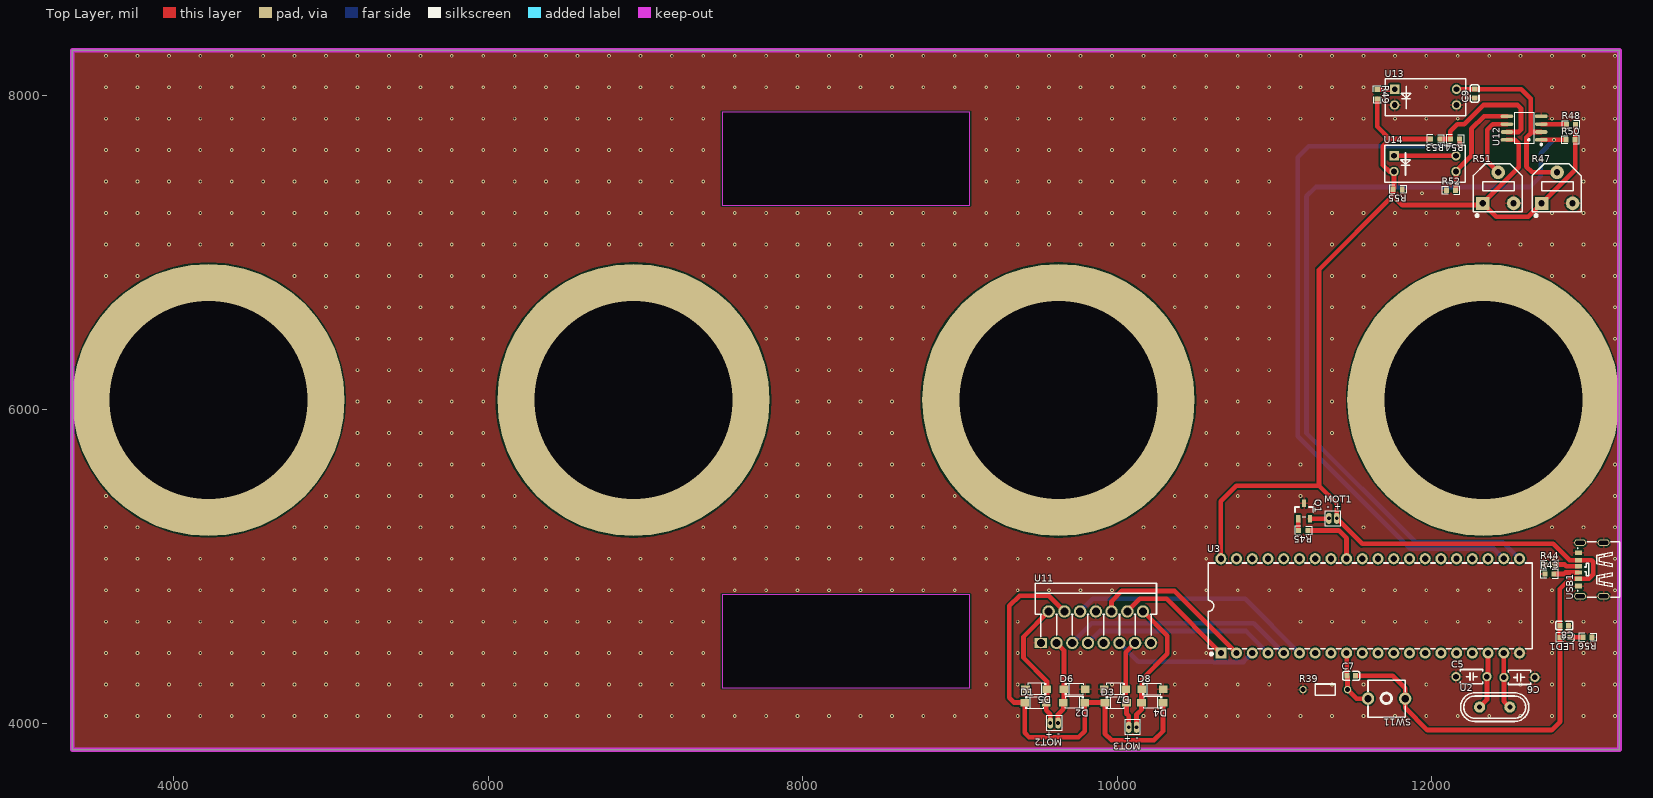
[diagram p0: Top Layer view]
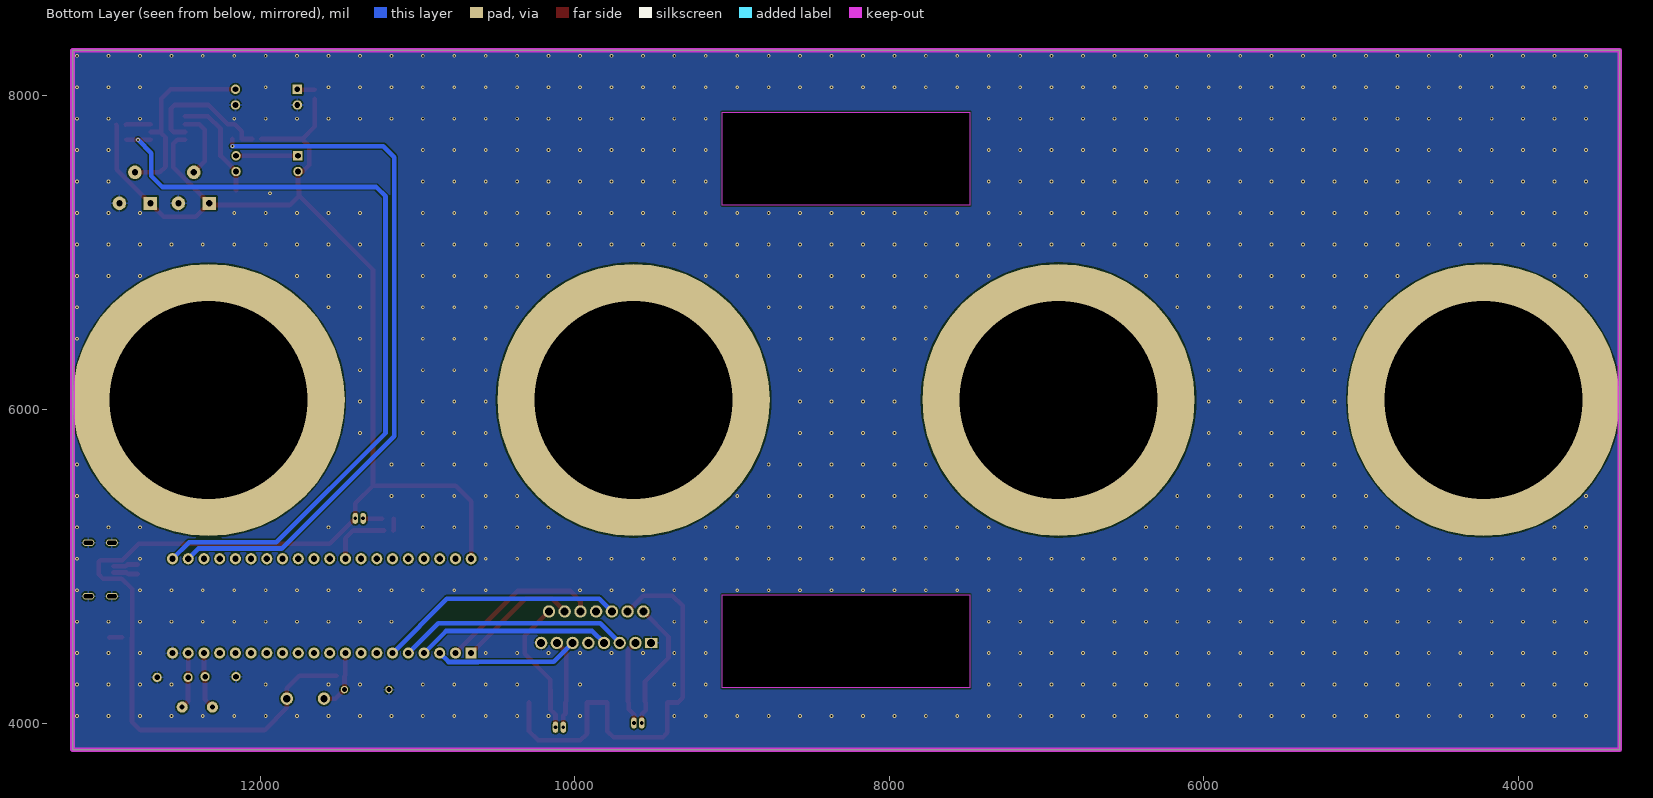
[diagram p1: Bottom Layer view, seen from below]
# Altium PCB MISC61231.pcbdoc
Units mil, origin at the board's own origin, x right, y up, seen from the top; angles counter-clockwise.
Board outline 9842.52 x 4448.82 mil, 2 copper layers (Top Layer, Bottom Layer), stack 62.206 mil thick; 40 components, 32 nets, 156 pads, 697 vias.

## Layer stack, top to bottom
Top Solder Mask Layer: solder mask 0.394, Dk 3.3
Top Layer: signal copper 1.379
SUBSTRATE1: surface 59.449, FR4, Dk 4.5
Bottom Layer: signal copper 1.378
Bottom Solder Mask Layer: solder mask 0.394, Dk 3.3

## Board outline
3353.74,8284.41 3353.74,3835.59 13196.26,3835.59 13196.26,8284.41
cut-out: 7487.6,7890.71 7487.6,7300.16 9062.4,7300.16 9062.4,7890.71
cut-out: 9062.4,4229.29 9062.4,4819.84 7487.6,4819.84 7487.6,4229.29

## Design rules (kind name [scope] priority, off if disabled: settings)
BoardOutlineClearance copperThickness2oz_1 [All] p2 off: genericclearance=7.99 ignorepadtopadclearanceinfootprint=FALSE except(0: Arc-SplitContinuation Track-SplitContinuation SMDPad-SplitContinuation THPad-SplitContinuation Via-SplitContinuation Fill-SplitContinuation Region-SplitContinuation Poly-SplitContinuation Text-SplitContinuation Hole-SplitContinuation; 5.98: Arc-CutoutEdge Track-CutoutEdge SMDPad-CutoutEdge THPad-CutoutEdge Via-CutoutEdge Text-CutoutEdge; 6.9: Hole-OutlineEdge Hole-CutoutEdge; 10: Poly-OutlineEdge Poly-CutoutEdge; 11.81: Arc-OutlineEdge Track-OutlineEdge SMDPad-OutlineEdge THPad-OutlineEdge Via-OutlineEdge Fill-OutlineEdge Region-OutlineEdge Text-OutlineEdge Fill-CutoutEdge Region-CutoutEdge)
BoardOutlineClearance Plane_innerPlane_1 [All] p4 off: genericclearance=4.02 ignorepadtopadclearanceinfootprint=FALSE except(0: Arc-SplitContinuation Track-SplitContinuation SMDPad-SplitContinuation THPad-SplitContinuation Via-SplitContinuation Fill-SplitContinuation Region-SplitContinuation Poly-SplitContinuation Text-SplitContinuation Hole-SplitContinuation; 5.98: Arc-CutoutEdge Track-CutoutEdge SMDPad-CutoutEdge THPad-CutoutEdge Via-CutoutEdge Text-CutoutEdge; 6.9: Hole-OutlineEdge Hole-CutoutEdge; 10: Poly-OutlineEdge Poly-CutoutEdge; 11.81: Arc-OutlineEdge Track-OutlineEdge SMDPad-OutlineEdge THPad-OutlineEdge Via-OutlineEdge Fill-OutlineEdge Region-OutlineEdge Text-OutlineEdge Fill-CutoutEdge Region-CutoutEdge)
BoardOutlineClearance Copper_copperRegion_1 [All] p6 off: genericclearance=4.02 ignorepadtopadclearanceinfootprint=FALSE except(0: Arc-SplitContinuation Track-SplitContinuation SMDPad-SplitContinuation THPad-SplitContinuation Via-SplitContinuation Fill-SplitContinuation Region-SplitContinuation Poly-SplitContinuation Text-SplitContinuation Hole-SplitContinuation; 5.98: Arc-CutoutEdge Track-CutoutEdge SMDPad-CutoutEdge THPad-CutoutEdge Via-CutoutEdge Text-CutoutEdge; 6.9: Hole-OutlineEdge Hole-CutoutEdge; 10: Poly-OutlineEdge Poly-CutoutEdge; 11.81: Arc-OutlineEdge Track-OutlineEdge SMDPad-OutlineEdge THPad-OutlineEdge Via-OutlineEdge Fill-OutlineEdge Region-OutlineEdge Text-OutlineEdge Fill-CutoutEdge Region-CutoutEdge)
BoardOutlineClearance copperThickness1oz_1 [All] p8: genericclearance=4.02 ignorepadtopadclearanceinfootprint=FALSE except(0: Arc-SplitContinuation Track-SplitContinuation SMDPad-SplitContinuation THPad-SplitContinuation Via-SplitContinuation Fill-SplitContinuation Region-SplitContinuation Poly-SplitContinuation Text-SplitContinuation Hole-SplitContinuation; 5.98: Arc-CutoutEdge Track-CutoutEdge SMDPad-CutoutEdge THPad-CutoutEdge Via-CutoutEdge Text-CutoutEdge; 6.9: Hole-OutlineEdge Hole-CutoutEdge; 10: Poly-OutlineEdge Poly-CutoutEdge; 11.81: Arc-OutlineEdge Track-OutlineEdge SMDPad-OutlineEdge THPad-OutlineEdge Via-OutlineEdge Fill-OutlineEdge Region-OutlineEdge Text-OutlineEdge Fill-CutoutEdge Region-CutoutEdge)
Clearance copperThickness2oz [All] p1 off: gap=7.99 ignorepadtopadclearanceinfootprint=FALSE except(5.98: SMDPad-Track SMDPad-SMDPad THPad-Track SMDPad-THPad THPad-THPad Track-Via SMDPad-Via THPad-Via Via-Via Fill-SMDPad Region-SMDPad Fill-THPad Region-THPad Fill-Via Region-Via Fill-Fill Fill-Region Region-Region Arc-Track Arc-SMDPad Arc-THPad Arc-Via Fill-Arc Region-Arc Arc-Arc Text-Track SMDPad-Text Text-THPad Text-Via Fill-Text Region-Text Arc-Text Text-Text; 6.9: Hole-Track Hole-SMDPad Hole-THPad Hole-Via Fill-Hole Region-Hole Hole-Arc Hole-Text; 10: Poly-Track Poly-SMDPad Poly-THPad Poly-Via Poly-Fill Poly-Region Poly-Poly Poly-Arc Poly-Text Poly-Hole; 11.81: Fill-Track Region-Track)
Clearance Plane_innerPlane [All] p3 off: gap=4.02 ignorepadtopadclearanceinfootprint=FALSE except(5.98: SMDPad-Track SMDPad-SMDPad THPad-Track SMDPad-THPad THPad-THPad Track-Via SMDPad-Via THPad-Via Via-Via Fill-SMDPad Region-SMDPad Fill-THPad Region-THPad Fill-Via Region-Via Fill-Fill Fill-Region Region-Region Arc-Track Arc-SMDPad Arc-THPad Arc-Via Fill-Arc Region-Arc Arc-Arc Text-Track SMDPad-Text Text-THPad Text-Via Fill-Text Region-Text Arc-Text Text-Text; 6.9: Hole-Track Hole-SMDPad Hole-THPad Hole-Via Fill-Hole Region-Hole Hole-Arc Hole-Text; 10: Poly-Track Poly-SMDPad Poly-THPad Poly-Via Poly-Fill Poly-Region Poly-Poly Poly-Arc Poly-Text Poly-Hole; 11.81: Fill-Track Region-Track)
Clearance Copper_copperRegion [All] p5 off: gap=4.02 ignorepadtopadclearanceinfootprint=FALSE except(5.98: SMDPad-Track SMDPad-SMDPad THPad-Track SMDPad-THPad THPad-THPad Track-Via SMDPad-Via THPad-Via Via-Via Fill-SMDPad Region-SMDPad Fill-THPad Region-THPad Fill-Via Region-Via Fill-Fill Fill-Region Region-Region Arc-Track Arc-SMDPad Arc-THPad Arc-Via Fill-Arc Region-Arc Arc-Arc Text-Track SMDPad-Text Text-THPad Text-Via Fill-Text Region-Text Arc-Text Text-Text; 6.9: Hole-Track Hole-SMDPad Hole-THPad Hole-Via Fill-Hole Region-Hole Hole-Arc Hole-Text; 10: Poly-Track Poly-SMDPad Poly-THPad Poly-Via Poly-Fill Poly-Region Poly-Poly Poly-Arc Poly-Text Poly-Hole; 11.81: Fill-Track Region-Track)
Clearance copperThickness1oz [All] p7: gap=4.02 ignorepadtopadclearanceinfootprint=FALSE except(5.98: SMDPad-Track SMDPad-SMDPad THPad-Track SMDPad-THPad THPad-THPad Track-Via SMDPad-Via THPad-Via Via-Via Fill-SMDPad Region-SMDPad Fill-THPad Region-THPad Fill-Via Region-Via Fill-Fill Fill-Region Region-Region Arc-Track Arc-SMDPad Arc-THPad Arc-Via Fill-Arc Region-Arc Arc-Arc Text-Track SMDPad-Text Text-THPad Text-Via Fill-Text Region-Text Arc-Text Text-Text; 6.9: Hole-Track Hole-SMDPad Hole-THPad Hole-Via Fill-Hole Region-Hole Hole-Arc Hole-Text; 10: Poly-Track Poly-SMDPad Poly-THPad Poly-Via Poly-Fill Poly-Region Poly-Poly Poly-Arc Poly-Text Poly-Hole; 11.81: Fill-Track Region-Track)
DiffPairsRouting differentialPair [All] p1: maxlimit=6 minlimit=6 mostfreqgap=6 toplayer_minwidth=5 toplayer_prefwidth=10 toplayer_maxwidth=100 toplayer_mingap=6 toplayer_prefgap=6 toplayer_maxgap=6 bottomlayer_minwidth=5 bottomlayer_prefwidth=10 bottomlayer_maxwidth=100 bottomlayer_mingap=6 bottomlayer_prefgap=6 bottomlayer_maxgap=6 maxuncoupledlength=10
HoleToHoleClearance otherClearance [All] p1: gap=11.81 allowstackedmicrovias=TRUE
Length netLength [All] p1: minlimit=0 maxlimit=0
PasteMaskExpansion pasteMaskExpansion [All] p1: expansion=0
PlaneConnect innerPlane [All] p1: planeconnectstyle=Relief reliefexpansion=20 reliefentries=4 reliefconductorwidth=10 reliefairgap=10
PolygonConnect copperRegion [All] p1: connectstyle=Relief reliefconductorwidth=10 reliefentries=4 polygonreliefangle="90 Angle" airgapwidth=10 via.connectstyle=Relief via.reliefconductorwidth=10 via.reliefentries=4 via.polygonreliefangle="90 Angle" via.airgapwidth=10
RoutingVias viaSize [All] p1: holewidth=12.01 width=24.02 viastyle="Through Hole" minholewidth=11.81 minwidth=19.68 maxholewidth=248.03 maxwidth=393.7
SolderMaskExpansion solderMaskExpansion [IsVia] p1: expansion=-1000 istentingtop=TRUE
SolderMaskExpansion solderMaskExpansion [All] p2: expansion=2 istentingtop=FALSE
Width copperThickness2oz_2 [All] p1 off: maxlimit=100 minlimit=8 preferedwidth=10
Width copperThickness1oz_2 [All] p2: maxlimit=100 minlimit=5 preferedwidth=10

## Components (designator, comment, footprint, x,y, rotation, side; value= is the part's Value field where it differs from the comment)
C5 "22pF" CAP-TH_L3.6-W2.3-P5.00-D0.5 12255,4300 r0 top
C6 "22pF" CAP-TH_L3.6-W2.3-P5.00-D0.5 12560,4295 r180 top
C7 "100pF" C0603 11490,4305 r0 top
C8 "100nF" C0603 12845,4625 r180 top
C9 "100nF" C0603 12275,8010 r90 top
D1 "" SOD-123FL_L2.7-W1.8-LS3.8-RD 9480.6,4134.85 r0 top
D2 "" SOD-123FL_L2.7-W1.8-LS3.8-RD 9725.6,4134.85 r180 top
D3 "" SOD-123FL_L2.7-W1.8-LS3.8-RD 9991.7,4134.85 r0 top
D4 "" SOD-123FL_L2.7-W1.8-LS3.8-RD 10224.2,4134.85 r180 top
D5 "" SOD-123FL_L2.7-W1.8-LS3.8-RD 9485.6,4219.85 r180 top
D6 "" SOD-123FL_L2.7-W1.8-LS3.8-RD 9730.6,4219.85 r0 top
D7 "" SOD-123FL_L2.7-W1.8-LS3.8-RD 9986.7,4219.85 r180 top
D8 "" SOD-123FL_L2.7-W1.8-LS3.8-RD 10225,4220 r0 top
LED1 "" LED_0603 12848.12,4549.5 r180 top
MOT1 "LCM1027A2445F" VIBRATING-MOTOR-SMD_WELDING 11372.83,5306.98 r0 top
MOT2 "LCM1027A2445F" VIBRATING-MOTOR-SMD_WELDING 9600,4005 r180 top
MOT3 "LCM1027A2445F" VIBRATING-MOTOR-SMD_WELDING 10099.2,3978.1 r180 top
Q1 "" S8550P_SOT 11190,5355 r270 top
R39 "10kΩ" Res_1/8W 11325,4215 r0 top
R43 "5.1K" R0603 12751.74,4952.71 r0 top
R44 "5.1K" R0603 12751.4,5012.79 r0 top
R45 "1K" R0603 11185,5230 r180 top
R47 "10kΩ" RES-ADJ-SMD_RM065-V1 12800,7410 r0 top
R48 "10K" R0603 12888.01,7811.59 r0 top
R49 "100K" R0603 11655,8005 r270 top
R50 "10K" R0603 12885,7715 r0 top
R51 "10kΩ" RES-ADJ-SMD_RM065-V1 12425,7410 r0 top
R52 "47K" R0603 12125,7395 r0 top
R53 "10K" R0603 12025,7720 r180 top
R54 "1K" R0603 12150,7720 r180 top
R55 "10K" R0603 11785,7400 r180 top
R56 "1K" R0603 12993.12,4549.5 r180 top
SW11 "Tactile switch, 6*6*5 plastic head, 260G, travel 0.25mm, through-hole 2-pin" KEY-TH_2P-L6.0-W6.0-P5.00 11715,4160 r180 top
U2 "12MHz" HC-49US_L11.0-W4.6-P4.88 12402.98,4105.88 r0 top
U3 "AT89C51" DIP-40_L52.3-W13.9-P2.54-LS15.2-BL 11610.62,4749.94 r0 top
U11 "L298N" MULTIWATT-15_L19.6-W5.0-P1.27-L 9865.27,4614.52 r0 top
U12 "LM393M" SOIC-8_L4.9-W3.9-P1.27-LS6.0-BL 12590,7790 r90 top
U13 "XL-ITR9707" OPTO-TH_4P-P2.54-XL-ITR9608 11963.01,7986.74 r0 top
U14 "XL-ITR9707" OPTO-TH_4P-P2.54-XL-ITR9608 11959.39,7563.75 r0 top
USB1 "TYPE_C_SMD_6P" TYPE-C-SMD_TYPE-C-6P 13015.67,4981.84 r90 top

## Footprints (in the part's own frame and the unit in brackets; to place one, negate y for a bottom-side part, rotate by r counter-clockwise, add the part's x,y. Pads: shape width x height; smd on the part's side, far side on the other; paste and mask are expansions set on the pad)
C0603 [mm]
  rect 0.8x0.9 smd: 1(-0.7,0) 2(0.7,0)
  silkscreen extent -1.39,-0.71 1.39,0.71
CAP-TH_L3.6-W2.3-P5.00-D0.5 [mm]
  round 1.5 hole 0.9: 1(-2.5,0) 2(2.5,0)
  silkscreen extent -1.8,-1.15 1.8,1.15
DIP-40_L52.3-W13.9-P2.54-LS15.2-BL [mm]
  rect 1.8x1.8 hole 1: 1(-24.13,-7.62)
  round 1.8 hole 1: 2(-21.59,-7.62) 3(-19.05,-7.62) 4(-16.51,-7.62) 5(-13.97,-7.62) 6(-11.43,-7.62) 7(-8.89,-7.62) 8(-6.35,-7.62) 9(-3.81,-7.62) 10(-1.27,-7.62) 11(1.27,-7.62) 12(3.81,-7.62) 13(6.35,-7.62) 14(8.89,-7.62) 15(11.43,-7.62) 16(13.97,-7.62) 17(16.51,-7.62) 18(19.05,-7.62) 19(21.59,-7.62) 20(24.13,-7.62) 21(24.13,7.62) 22(21.59,7.62) 23(19.05,7.62) 24(16.51,7.62) 25(13.97,7.62) 26(11.43,7.62) 27(8.89,7.62) 28(6.35,7.62) 29(3.81,7.62) 30(1.27,7.62) 31(-1.27,7.62) 32(-3.81,7.62) 33(-6.35,7.62) 34(-8.89,7.62) 35(-11.43,7.62) 36(-13.97,7.62) 37(-16.51,7.62) 38(-19.05,7.62) 39(-21.59,7.62) 40(-24.13,7.62)
  silkscreen extent -26.16,-7.95 26.16,6.93
HC-49US_L11.0-W4.6-P4.88 [mm]
  round 1.8 hole 0.8: 1(-2.44,0) 2(2.44,0)
  silkscreen extent -5.51,-2.32 5.51,2.32
KEY-TH_2P-L6.0-W6.0-P5.00 [mm]
  round 2 hole 1.2: 1(-3,0) 2(3,0)
  silkscreen extent -3,-3 3,3
LED_0603 [mil]
  rect 31.5x31.5 smd paste+0 mask+2: 1(-33.5,-0.4) 2(29.5,-0.2)
  silkscreen extent -61,-30 53,30
MULTIWATT-15_L19.6-W5.0-P1.27-L [mm]
  rect 2x1.6 hole 1.3 paste+0 mask+0.051: 1(-8.89,-2.54)
  round 2 hole 1.3 paste+0 mask+0.051: 2(-7.62,2.54) 3(-6.35,-2.54) 4(-5.08,2.54) 5(-3.81,-2.54) 6(-2.54,2.54) 7(-1.27,-2.54) 8(0,2.54) 9(1.27,-2.54) 10(2.54,2.54) 11(3.81,-2.54) 12(5.08,2.54) 13(6.35,-2.54) 14(7.62,2.54) 15(8.89,-2.54)
  silkscreen extent -9.8,-1.52 9.8,7.09
OPTO-TH_4P-P2.54-XL-ITR9608 [mil]
  rect 60x60 hole 36: 1(-196.85,50)
  round 60 hole 36: 2(-196.85,-50) 3(196.85,-50) 4(196.84,50)
  silkscreen extent -256,-118 256,118
R0603 [mil]
  rect 31.75x34.02 smd paste-3937.01 mask+2: 1(-29.66,0) 2(29.66,0)
  silkscreen extent -55,-26 55,26
RES-ADJ-SMD_RM065-V1 [mm]
  rect 2.2x2.1 hole 1 paste+0 mask+0.05: 1(-2.5,-2.5)
  round 2.2 hole 1 paste+0 mask+0.05: 2(0,2.5) 3(2.5,-2.5)
  silkscreen extent -4,-4.7 3.9,3.9
Res_1/8W [mil]
  round 47.2 hole 31.5 paste+0 mask+2: 1(-141.7,2.48) 2(141.7,2.48)
  silkscreen extent -63,-33 63,38
S8550P_SOT [mil]
  rect 49.2x27.6 smd paste+0 mask+2: 1(50.84,-37.4) 2(50.84,37.4) 3(-47.56,0)
  silkscreen extent -24,-58 37,58
SOD-123FL_L2.7-W1.8-LS3.8-RD [mil]
  rect 55.1x47.2 smd paste+0 mask+2: 1(-68.3,0) 2(68.3,0)
  silkscreen extent -63,-39 54,40
SOIC-8_L4.9-W3.9-P1.27-LS6.0-BL [mm]
  oval 0.588x2.045 smd: 1(-1.905,-2.772) 2(-0.635,-2.772) 3(0.635,-2.772) 4(1.905,-2.772) 5(1.905,2.772) 6(0.635,2.772) 7(-0.635,2.772) 8(-1.905,2.772)
  silkscreen extent -2.8,-2.92 2.53,1.52
TYPE-C-SMD_TYPE-C-6P [mm]
  oval 1.1x1.9 hole 0.7 slot 1.5 at 90 deg: 7(-4.32,-2.025) 7(-4.32,1.775) 7(4.32,-2.025) 7(4.32,1.775)
  rect 0.7x1.2 smd paste-100 mask+0.051: A5(-0.5,2.025) A9(1.5,2.025) B5(0.5,2.025) B9(-1.5,2.025)
  rect 0.8x1.2 smd paste-100 mask+0.051: A12(2.7,2.025) B12(-2.7,2.025)
  silkscreen extent -4.5,-4.63 4.5,2.18
VIBRATING-MOTOR-SMD_WELDING [mm]
  oval 0.9x1.8 hole 0.61 paste+0 mask+0.05: 1(-0.635,0) 2(0.635,0)
  silkscreen extent -1.27,-1.17 1.27,1.17

## Free pads (board coordinates)
  round 1732.28 hole 1259.84: 1(4219.88,6060) 1(6923.29,6060) 1(9626.71,6060) 1(12330.12,6060)

## Via types
v1: diameter 24.02, hole 12, Top Layer to Bottom Layer, 697 vias

## Nets (pads, with @x,y where several pads share a name; then routed paths per layer and width w, separated by ;. In a path a pad name is that pad's centre, name@x,y a point inside that pad or via, vN(x,y) a via of type N, cw(c..) or ccw(c..) an arc to the next point about the centre after c; other vN are vias at no path point)
12V: D1.1 D2.1 D3.1 D4.1 U11.4 | length 2816.2
  Top Layer w30: U11.4 9564.79,4815 9380,4815 9315,4750 9315,4164.85 9345,4134.85 D1.1 9412.3,3942.7 9440,3915 9755,3915 9793.9,3953.9 D2.1 D3.1 9923.4,3936.6 9965,3895 10235,3895 10292.5,3952.5 D4.1
$1N1611: C5.2 U2.1 U3.18 | length 366.3
  Top Layer w30: U2.1 12353.42,4152.39 C5.2 12360.62,4307.19 U3.18
$1N1612: C6.2 U2.2 U3.19 | length 360
  Top Layer w30: U3.19 12460.62,4295.96 C6.2 12461.58,4143.35 U2.2
$1N1662: C7.1 R39.2 SW11.2 U3.9 | length 389
  Top Layer w30: U3.9 11462.44,4448.12 C7.1 11466.7,4300.74 R39.2 11524.18,4160 SW11.2
$1N14764: R43.2 USB1.A5 | length 158.5
  Top Layer w30: R43.2 12842.71,4952.71 12852.15,4962.15 USB1.A5
$1N14769: R44.2 USB1.B5 | length 159.6
  Top Layer w30: R44.2 12847.21,5012.79 12858.48,5001.52 USB1.B5
$1N18211: R45.1 U3.32 | length 396.4
  Top Layer w30: R45.1 11410,5230 11460.62,5179.38 U3.32
$1N18265: Q1.1 R45.2 | length 75.3
  Top Layer w30: Q1.1 11152.6,5232.74 R45.2
$1N18397: MOT1.1 Q1.2 | length 121.6
  Top Layer w30: Q1.2 11345.02,5304.16 MOT1.1
$1N19527: D1.2 D5.1 MOT2.2 U11.2 | length 850.5
  Top Layer w30: U11.2 9405,4554.26 9405,4420 9553.9,4271.1 D5.1 9553.9,4139.85 D1.2 9548.9,4086.1 9575,4060 MOT2.2
$1N19528: D2.2 D6.1 MOT2.1 U11.3 | length 544.5
  Top Layer w30: U11.3 9662.3,4467.5 D6.1 9662.3,4139.85 D2.2 9657.3,4092.3 9625,4060 MOT2.1
$1N19534: D3.2 D7.1 MOT3.2 U11.13 | length 569.3
  Top Layer w30: MOT3.2 10074.2,4050.8 10060,4065 D3.2 10055,4139.85 D7.1 10055,4454.25 U11.13
$1N19535: D4.2 D8.1 MOT3.1 U11.14 | length 881.6
  Top Layer w30: MOT3.1 10124.2,4059.2 10155.9,4090.9 D4.2 10155.9,4219.2 D8.1 10156.7,4281.7 10320,4445 10320,4559.79 U11.14
$1N20827: C9.2 R47.2 U12.2 U13.4 | length 1221.8
  Top Layer w30: U13.4 12274.18,8036.74 C9.2 12572.44,8037.56 12632.32,7977.68 12632.32,7757.32 ; U12.2 12640,7765 12632.32,7757.32 ; R47.2 12641.58,7508.43 12605,7545 12605,7730 12632.32,7757.32
$1N20831: R48.1 U12.3 | length 160.6
  Top Layer w30: U12.3 12854.93,7815 R48.1
$1N20958: R49.1 U13.1 | length 112
  Top Layer w30: R49.1 11764.07,8034.66 U13.1
$1N21237: R52.2 U12.5 U14.3 | length 690.5
  Top Layer w30: R52.2 12156.25,7396.59 U14.3 12255,7612.5 12255,7785 12335,7865 U12.5
$1N21244: U14.1 U14.4 | length 393.7
  Top Layer w30: U14.1 U14.4
$1N21331: R51.2 U12.6 | length 440.9
  Top Layer w30: R51.2 12355,7578.43 12355,7780 12390,7815 U12.6
$1N21478: R53.1 R54.2 U12.7 | length 873.5
  Top Layer w30: R53.1 R54.2 12120.34,7770.34 12165,7815 12210,7815 12331.21,7936.21 12548.79,7936.21 12570,7915 12570,7780 12555,7765 U12.7
$1N21618: LED1.1 R56.2 | length 82
  Top Layer w30: LED1.1 12963.06,4549.9 R56.2
+5V: U11.9
BIZHANG: R50.1 U3.21 U12.1 | length 5157.3
  Top Layer w30: U12.1 v1(12780,7715) R50.1
  Bottom Layer w30: U3.21 12455.56,5155 11900,5155 11205,5850 11205,7355 11265,7415 12625,7415 12695,7485 12695,7630 v1(12780,7715)
EA: U3.6 U11.6 | length 1571.6
  Bottom Layer w30: U11.6 9845.74,4795 10815.56,4795 U3.6
EB: U3.3 U11.11 | length 918.8
  Bottom Layer w30: U11.11 10134.79,4395 10615.02,4395 10616.49,4393.52 10804.2,4393.52 U3.3
FANGDIELUO: R54.1 U3.22 | length 4512.4
  Top Layer w30: v1(12179.66,7675) R54.1
  Bottom Layer w30: v1(12179.66,7675) 11220,7675 11150,7605 11150,5830 11865,5115 12395.56,5115 U3.22
GND: C5.1 C6.1 C8.1 C9.1 D5.2 D6.2 D7.2 D8.2 Q1.3 R39.1 R43.1 R44.1 R47.3 R51.3 R52.1 R55.1 R56.1 U3.20 U11.1 U11.8 U11.15 U12.4 U13.2 U13.3 USB1.7 USB1.A12 USB1.B12
  other v1: 3567.84,4049.69 3767.84,4049.69 3967.84,4049.69 4167.84,4049.69 4367.84,4049.69 4567.84,4049.69 4767.84,4049.69 4967.84,4049.69 5167.84,4049.69 5367.84,4049.69 5567.84,4049.69 5767.84,4049.69 5967.84,4049.69 6167.84,4049.69 6367.84,4049.69 6567.84,4049.69 6767.84,4049.69 6967.84,4049.69 7167.84,4049.69 7367.84,4049.69 7567.84,4049.69 7767.84,4049.69 7967.84,4049.69 8167.84,4049.69 8367.84,4049.69 8567.84,4049.69 8767.84,4049.69 8967.84,4049.69 9167.84,4049.69 9367.84,4049.69 9967.84,4049.69 10167.84,4049.69 10367.84,4049.69 10567.84,4049.69 10767.84,4049.69 10967.84,4049.69 11167.84,4049.69 11367.84,4049.69 11567.84,4049.69 11767.84,4049.69 11967.84,4049.69 12167.84,4049.69 12367.84,4049.69 12567.84,4049.69 12767.84,4049.69 12967.84,4049.69 13167.84,4049.69 3567.84,4249.69 3767.84,4249.69 3967.84,4249.69 4167.84,4249.69 4367.84,4249.69 4567.84,4249.69 4767.84,4249.69 4967.84,4249.69 5167.84,4249.69 5367.84,4249.69 5567.84,4249.69 5767.84,4249.69 5967.84,4249.69 6167.84,4249.69 6367.84,4249.69 6567.84,4249.69 6767.84,4249.69 6967.84,4249.69 7167.84,4249.69 7367.84,4249.69 9167.84,4249.69 9367.84,4249.69 9967.84,4249.69 10367.84,4249.69 10567.84,4249.69 10767.84,4249.69 10967.84,4249.69 11367.84,4249.69 11567.84,4249.69 11967.84,4249.69 12567.84,4249.69 12767.84,4249.69 12967.84,4249.69 13167.84,4249.69 3567.84,4449.69 3767.84,4449.69 3967.84,4449.69 4167.84,4449.69 4367.84,4449.69 4567.84,4449.69 4767.84,4449.69 4967.84,4449.69 5167.84,4449.69 5367.84,4449.69 5567.84,4449.69 5767.84,4449.69 5967.84,4449.69 6167.84,4449.69 6367.84,4449.69 6567.84,4449.69 6767.84,4449.69 6967.84,4449.69 7167.84,4449.69 7367.84,4449.69 9167.84,4449.69 9367.84,4449.69 9567.84,4449.69 9767.84,4449.69 9967.84,4449.69 10167.84,4449.69 10367.84,4449.69 10567.84,4449.69 12767.84,4449.69 12967.84,4449.69 13167.84,4449.69 3567.84,4649.69 3767.84,4649.69 3967.84,4649.69 4167.84,4649.69 4367.84,4649.69 4567.84,4649.69 4767.84,4649.69 4967.84,4649.69 5167.84,4649.69 5367.84,4649.69 5567.84,4649.69 5767.84,4649.69 5967.84,4649.69 6167.84,4649.69 6367.84,4649.69 6567.84,4649.69 6767.84,4649.69 6967.84,4649.69 7167.84,4649.69 7367.84,4649.69 9167.84,4649.69 9367.84,4649.69 11167.84,4649.69 11367.84,4649.69 11567.84,4649.69 11767.84,4649.69 11967.84,4649.69 12167.84,4649.69 12367.84,4649.69 12567.84,4649.69 12767.84,4649.69 12967.84,4649.69 13167.84,4649.69 3567.84,4849.69 3767.84,4849.69 3967.84,4849.69 4167.84,4849.69 4367.84,4849.69 4567.84,4849.69 4767.84,4849.69 4967.84,4849.69 5167.84,4849.69 5367.84,4849.69 5567.84,4849.69 5767.84,4849.69 5967.84,4849.69 6167.84,4849.69 6367.84,4849.69 6567.84,4849.69 6767.84,4849.69 6967.84,4849.69 7167.84,4849.69 7367.84,4849.69 7567.84,4849.69 7767.84,4849.69 7967.84,4849.69 8167.84,4849.69 8367.84,4849.69 8567.84,4849.69 8767.84,4849.69 8967.84,4849.69 9167.84,4849.69 9367.84,4849.69 9567.84,4849.69 9767.84,4849.69 9967.84,4849.69 10567.84,4849.69 10767.84,4849.69 10967.84,4849.69 11167.84,4849.69 11367.84,4849.69 11567.84,4849.69 11767.84,4849.69 11967.84,4849.69 12167.84,4849.69 12367.84,4849.69 12567.84,4849.69 12767.84,4849.69 13167.84,4849.69 3567.84,5049.69 3767.84,5049.69 3967.84,5049.69 4167.84,5049.69 4367.84,5049.69 4567.84,5049.69 4767.84,5049.69 4967.84,5049.69 5167.84,5049.69 5367.84,5049.69 5567.84,5049.69 5767.84,5049.69 5967.84,5049.69 6167.84,5049.69 6367.84,5049.69 6567.84,5049.69 6767.84,5049.69 6967.84,5049.69 7167.84,5049.69 7367.84,5049.69 7567.84,5049.69 7767.84,5049.69 7967.84,5049.69 8167.84,5049.69 8367.84,5049.69 8567.84,5049.69 8767.84,5049.69 8967.84,5049.69 9167.84,5049.69 9367.84,5049.69 9567.84,5049.69 9767.84,5049.69 9967.84,5049.69 10167.84,5049.69 10367.84,5049.69 10567.84,5049.69 12767.84,5049.69 13167.84,5049.69 3567.84,5249.69 3767.84,5249.69 4767.84,5249.69 4967.84,5249.69 5167.84,5249.69 5367.84,5249.69 5567.84,5249.69 5767.84,5249.69 5967.84,5249.69 6167.84,5249.69 6367.84,5249.69 7367.84,5249.69 7567.84,5249.69 7767.84,5249.69 7967.84,5249.69 8167.84,5249.69 8367.84,5249.69 8567.84,5249.69 8767.84,5249.69 8967.84,5249.69 9167.84,5249.69 10167.84,5249.69 10367.84,5249.69 10567.84,5249.69 10767.84,5249.69 10967.84,5249.69 11567.84,5249.69 12767.84,5249.69 12967.84,5249.69 13167.84,5249.69 3567.84,5449.69 4967.84,5449.69 5167.84,5449.69 5367.84,5449.69 5567.84,5449.69 5767.84,5449.69 5967.84,5449.69 6167.84,5449.69 7767.84,5449.69 7967.84,5449.69 8167.84,5449.69 8367.84,5449.69 8567.84,5449.69 8767.84,5449.69 8967.84,5449.69 10367.84,5449.69 10567.84,5449.69 10767.84,5449.69 10967.84,5449.69 11167.84,5449.69 13167.84,5449.69 5167.84,5649.69 5367.84,5649.69 5567.84,5649.69 5767.84,5649.69 5967.84,5649.69 7767.84,5649.69 7967.84,5649.69 8167.84,5649.69 8367.84,5649.69 8567.84,5649.69 8767.84,5649.69 10567.84,5649.69 10767.84,5649.69 10967.84,5649.69 11167.84,5649.69 13167.84,5649.69 5167.84,5849.69 5367.84,5849.69 5567.84,5849.69 5767.84,5849.69 5967.84,5849.69 7967.84,5849.69 8167.84,5849.69 8367.84,5849.69 8567.84,5849.69 10567.84,5849.69 10767.84,5849.69 10967.84,5849.69 11367.84,5849.69 5167.84,6049.69 5367.84,6049.69 5567.84,6049.69 5767.84,6049.69 5967.84,6049.69 7967.84,6049.69 8167.84,6049.69 8367.84,6049.69 8567.84,6049.69 10567.84,6049.69 10767.84,6049.69 10967.84,6049.69 11367.84,6049.69 5167.84,6249.69 5367.84,6249.69 5567.84,6249.69 5767.84,6249.69 5967.84,6249.69 7967.84,6249.69 8167.84,6249.69 8367.84,6249.69 8567.84,6249.69 10567.84,6249.69 10767.84,6249.69 10967.84,6249.69 11367.84,6249.69 5167.84,6449.69 5367.84,6449.69 5567.84,6449.69 5767.84,6449.69 5967.84,6449.69 7767.84,6449.69 7967.84,6449.69 8167.84,6449.69 8367.84,6449.69 8567.84,6449.69 8767.84,6449.69 10567.84,6449.69 10767.84,6449.69 10967.84,6449.69 11367.84,6449.69 13167.84,6449.69 4967.84,6649.69 5167.84,6649.69 5367.84,6649.69 5567.84,6649.69 5767.84,6649.69 5967.84,6649.69 6167.84,6649.69 7767.84,6649.69 7967.84,6649.69 8167.84,6649.69 8367.84,6649.69 8567.84,6649.69 8767.84,6649.69 10367.84,6649.69 10567.84,6649.69 10767.84,6649.69 10967.84,6649.69 11367.84,6649.69 11567.84,6649.69 13167.84,6649.69 3567.84,6849.69 3767.84,6849.69 4767.84,6849.69 4967.84,6849.69 5167.84,6849.69 5367.84,6849.69 5567.84,6849.69 5767.84,6849.69 5967.84,6849.69 6167.84,6849.69 6367.84,6849.69 7367.84,6849.69 7567.84,6849.69 7767.84,6849.69 7967.84,6849.69 8167.84,6849.69 8367.84,6849.69 8567.84,6849.69 8767.84,6849.69 8967.84,6849.69 9167.84,6849.69 10167.84,6849.69 10367.84,6849.69 10567.84,6849.69 10767.84,6849.69 10967.84,6849.69 11367.84,6849.69 11567.84,6849.69 11767.84,6849.69 12767.84,6849.69 12967.84,6849.69 13167.84,6849.69 3567.84,7049.69 3767.84,7049.69 3967.84,7049.69 4167.84,7049.69 4367.84,7049.69 4567.84,7049.69 4767.84,7049.69 4967.84,7049.69 5167.84,7049.69 5367.84,7049.69 5567.84,7049.69 5767.84,7049.69 5967.84,7049.69 6167.84,7049.69 6367.84,7049.69 6567.84,7049.69 6767.84,7049.69 6967.84,7049.69 7167.84,7049.69 7367.84,7049.69 7567.84,7049.69 7767.84,7049.69 7967.84,7049.69 8167.84,7049.69 8367.84,7049.69 8567.84,7049.69 8767.84,7049.69 8967.84,7049.69 9167.84,7049.69 9367.84,7049.69 9567.84,7049.69 9767.84,7049.69 9967.84,7049.69 10167.84,7049.69 10367.84,7049.69 10567.84,7049.69 10767.84,7049.69 10967.84,7049.69 11367.84,7049.69 11567.84,7049.69 11767.84,7049.69 11967.84,7049.69 12167.84,7049.69 12367.84,7049.69 12567.84,7049.69 12767.84,7049.69 12967.84,7049.69 13167.84,7049.69 3567.84,7249.69 3767.84,7249.69 3967.84,7249.69 4167.84,7249.69 4367.84,7249.69 4567.84,7249.69 4767.84,7249.69 4967.84,7249.69 5167.84,7249.69 5367.84,7249.69 5567.84,7249.69 5767.84,7249.69 5967.84,7249.69 6167.84,7249.69 6367.84,7249.69 6567.84,7249.69 6767.84,7249.69 6967.84,7249.69 7167.84,7249.69 7367.84,7249.69 7567.84,7249.69 7767.84,7249.69 7967.84,7249.69 8167.84,7249.69 8367.84,7249.69 8567.84,7249.69 8767.84,7249.69 8967.84,7249.69 9167.84,7249.69 9367.84,7249.69 9567.84,7249.69 9767.84,7249.69 9967.84,7249.69 10167.84,7249.69 10367.84,7249.69 10567.84,7249.69 10767.84,7249.69 10967.84,7249.69 11367.84,7249.69 11567.84,7249.69 11767.84,7249.69 11967.84,7249.69 12167.84,7249.69 12767.84,7249.69 12967.84,7249.69 13167.84,7249.69 11940,7375 3567.84,7449.69 3767.84,7449.69 3967.84,7449.69 4167.84,7449.69 4367.84,7449.69 4567.84,7449.69 4767.84,7449.69 4967.84,7449.69 5167.84,7449.69 5367.84,7449.69 5567.84,7449.69 5767.84,7449.69 5967.84,7449.69 6167.84,7449.69 6367.84,7449.69 6567.84,7449.69 6767.84,7449.69 6967.84,7449.69 7167.84,7449.69 7367.84,7449.69 9167.84,7449.69 9367.84,7449.69 9567.84,7449.69 9767.84,7449.69 9967.84,7449.69 10167.84,7449.69 10367.84,7449.69 10567.84,7449.69 10767.84,7449.69 10967.84,7449.69 12967.84,7449.69 13167.84,7449.69 3567.84,7649.69 3767.84,7649.69 3967.84,7649.69 4167.84,7649.69 4367.84,7649.69 4567.84,7649.69 4767.84,7649.69 4967.84,7649.69 5167.84,7649.69 5367.84,7649.69 5567.84,7649.69 5767.84,7649.69 5967.84,7649.69 6167.84,7649.69 6367.84,7649.69 6567.84,7649.69 6767.84,7649.69 6967.84,7649.69 7167.84,7649.69 7367.84,7649.69 9167.84,7649.69 9367.84,7649.69 9567.84,7649.69 9767.84,7649.69 9967.84,7649.69 10167.84,7649.69 10367.84,7649.69 10567.84,7649.69 10767.84,7649.69 10967.84,7649.69 12967.84,7649.69 13167.84,7649.69 3567.84,7849.69 3767.84,7849.69 3967.84,7849.69 4167.84,7849.69 4367.84,7849.69 4567.84,7849.69 4767.84,7849.69 4967.84,7849.69 5167.84,7849.69 5367.84,7849.69 5567.84,7849.69 5767.84,7849.69 5967.84,7849.69 6167.84,7849.69 6367.84,7849.69 6567.84,7849.69 6767.84,7849.69 6967.84,7849.69 7167.84,7849.69 7367.84,7849.69 9167.84,7849.69 9367.84,7849.69 9567.84,7849.69 9767.84,7849.69 9967.84,7849.69 10167.84,7849.69 10367.84,7849.69 10567.84,7849.69 10767.84,7849.69 10967.84,7849.69 11167.84,7849.69 11367.84,7849.69 11567.84,7849.69 11767.84,7849.69 11967.84,7849.69 12167.84,7849.69 12767.84,7849.69 12967.84,7849.69 13167.84,7849.69 3567.84,8049.69 3767.84,8049.69 3967.84,8049.69 4167.84,8049.69 4367.84,8049.69 4567.84,8049.69 4767.84,8049.69 4967.84,8049.69 5167.84,8049.69 5367.84,8049.69 5567.84,8049.69 5767.84,8049.69 5967.84,8049.69 6167.84,8049.69 6367.84,8049.69 6567.84,8049.69 6767.84,8049.69 6967.84,8049.69 7167.84,8049.69 7367.84,8049.69 7567.84,8049.69 7767.84,8049.69 7967.84,8049.69 8167.84,8049.69 8367.84,8049.69 8567.84,8049.69 8767.84,8049.69 8967.84,8049.69 9167.84,8049.69 9367.84,8049.69 9567.84,8049.69 9767.84,8049.69 9967.84,8049.69 10167.84,8049.69 10367.84,8049.69 10567.84,8049.69 10767.84,8049.69 10967.84,8049.69 11167.84,8049.69 11367.84,8049.69 11567.84,8049.69 11967.84,8049.69 12767.84,8049.69 12967.84,8049.69 13167.84,8049.69 3567.84,8249.69 3767.84,8249.69 3967.84,8249.69 4167.84,8249.69 4367.84,8249.69 4567.84,8249.69 4767.84,8249.69 4967.84,8249.69 5167.84,8249.69 5367.84,8249.69 5567.84,8249.69 5767.84,8249.69 5967.84,8249.69 6167.84,8249.69 6367.84,8249.69 6567.84,8249.69 6767.84,8249.69 6967.84,8249.69 7167.84,8249.69 7367.84,8249.69 7567.84,8249.69 7767.84,8249.69 7967.84,8249.69 8167.84,8249.69 8367.84,8249.69 8567.84,8249.69 8767.84,8249.69 8967.84,8249.69 9167.84,8249.69 9367.84,8249.69 9567.84,8249.69 9767.84,8249.69 9967.84,8249.69 10167.84,8249.69 10367.84,8249.69 10567.84,8249.69 10767.84,8249.69 10967.84,8249.69 11167.84,8249.69 11367.84,8249.69 11567.84,8249.69 11767.84,8249.69 11967.84,8249.69 12167.84,8249.69 12367.84,8249.69 12567.84,8249.69 12767.84,8249.69 12967.84,8249.69 13167.84,8249.69
IN1: U3.5 U11.5 | length 1476
  Bottom Layer w30: U11.5 9840.74,4640 10870.56,4640 U3.5
IN2: U3.4 U11.7 | length 1234.6
  Bottom Layer w30: U11.7 9890.74,4590 10820.56,4590 U3.4
IN3: U3.2 U11.10 | length 1051.9
  Top Layer w30: U11.10 9965.27,4780.27 10030,4845 10365.56,4845 10704.2,4506.36 10704.74,4506.36 10717.03,4494.07 10717.03,4493.52 U3.2
IN4: U3.1 U11.12 | length 771.6
  Top Layer w30: U11.12 10145.74,4795 10315.56,4795 U3.1
VCC: C7.2 C8.2 LED1.2 MOT1.2 R47.1 R48.2 R49.2 R50.2 R51.1 R53.2 R55.2 SW11.1 U3.40 U12.8 U14.2 USB1.A9 USB1.B9 | length 10949.3
  Top Layer w30: U3.40 10660.62,5415.62 10760,5515 11285,5515 ; C7.2 11755,4305 11833.11,4226.89 SW11.1 11833.11,4101.89 11975,3960 12765,3960 12818.62,4013.62 LED1.2 12817.44,4550.88 C8.2 12817.44,4857.44 12882.78,4922.78 USB1.B9 13002.78,4922.78 13030,4950 13030,5030 13019.11,5040.89 USB1.A9 12879.11,5040.89 12775,5145 11559.81,5145 MOT1.2 11397.83,5402.17 11285,5515 ; R49.2 11655,7800 11735,7720 ; R53.2 11735,7720 ; R51.1@12320,7300 11815,7300 11755.34,7359.66 ; U12.8 12530,7715 12555,7690 12555,7540 R51.1 12413.15,7225 12615,7225 R47.1 12914.66,7524.66 R50.2 12914.66,7808.58 R48.2 ; 11285,5515 11285,6889.32 11755.34,7359.66 ; 11735,7720 11690,7675 11690,7555 11731.25,7513.75 U14.2 11762.55,7407.21 R55.2 11755.34,7359.66
pads on no net: U3.7 U3.8 U3.10 U3.11 U3.12 U3.13 U3.14 U3.15 U3.16 U3.17 U3.23 U3.24 U3.25 U3.26 U3.27 U3.28 U3.29 U3.30 U3.31 U3.33 U3.34 U3.35 U3.36 U3.37 U3.38 U3.39

## Polygon pours and split planes (outlines as drawn)
GND on Top Layer (solid, remove dead copper, pour order 0): 3000,8950 3000,3425 13905,3425 13905,8950
GND on Bottom Layer (solid, remove dead copper, pour order 2): 3135,8640 3135,3000 14010,3000 14010,8640

## Keep-outs
Board Outline Layer:
  region: 7487.6,7890.71 7487.6,7300.16 9062.4,7300.16 9062.4,7890.71
  region: 7487.6,7890.71 7487.6,7300.16 9062.4,7300.16 9062.4,7890.71
  region: 9062.4,4229.29 9062.4,4819.84 7487.6,4819.84 7487.6,4229.29
  region: 9062.4,4229.29 9062.4,4819.84 7487.6,4819.84 7487.6,4229.29
  lines w0.1: 7487.6,4229.29 7487.6,4819.84 9062.4,4819.84 9062.4,4229.29 7487.6,4229.29 ; 7487.6,7300.16 7487.6,7890.71 9062.4,7890.71 9062.4,7300.16 7487.6,7300.16
  lines w30: 3353.74,3835.59 3353.74,8284.41 13196.26,8284.41 13196.26,3835.59 3353.74,3835.59

## Silkscreen, mask and mechanical layers (free items; w line width, h text height)
Mechanical Layer:
  lines w0.1: 7487.6,4229.29 7487.6,4819.84 9062.4,4819.84 9062.4,4229.29 7487.6,4229.29 ; 7487.6,7300.16 7487.6,7890.71 9062.4,7890.71 9062.4,7300.16 7487.6,7300.16